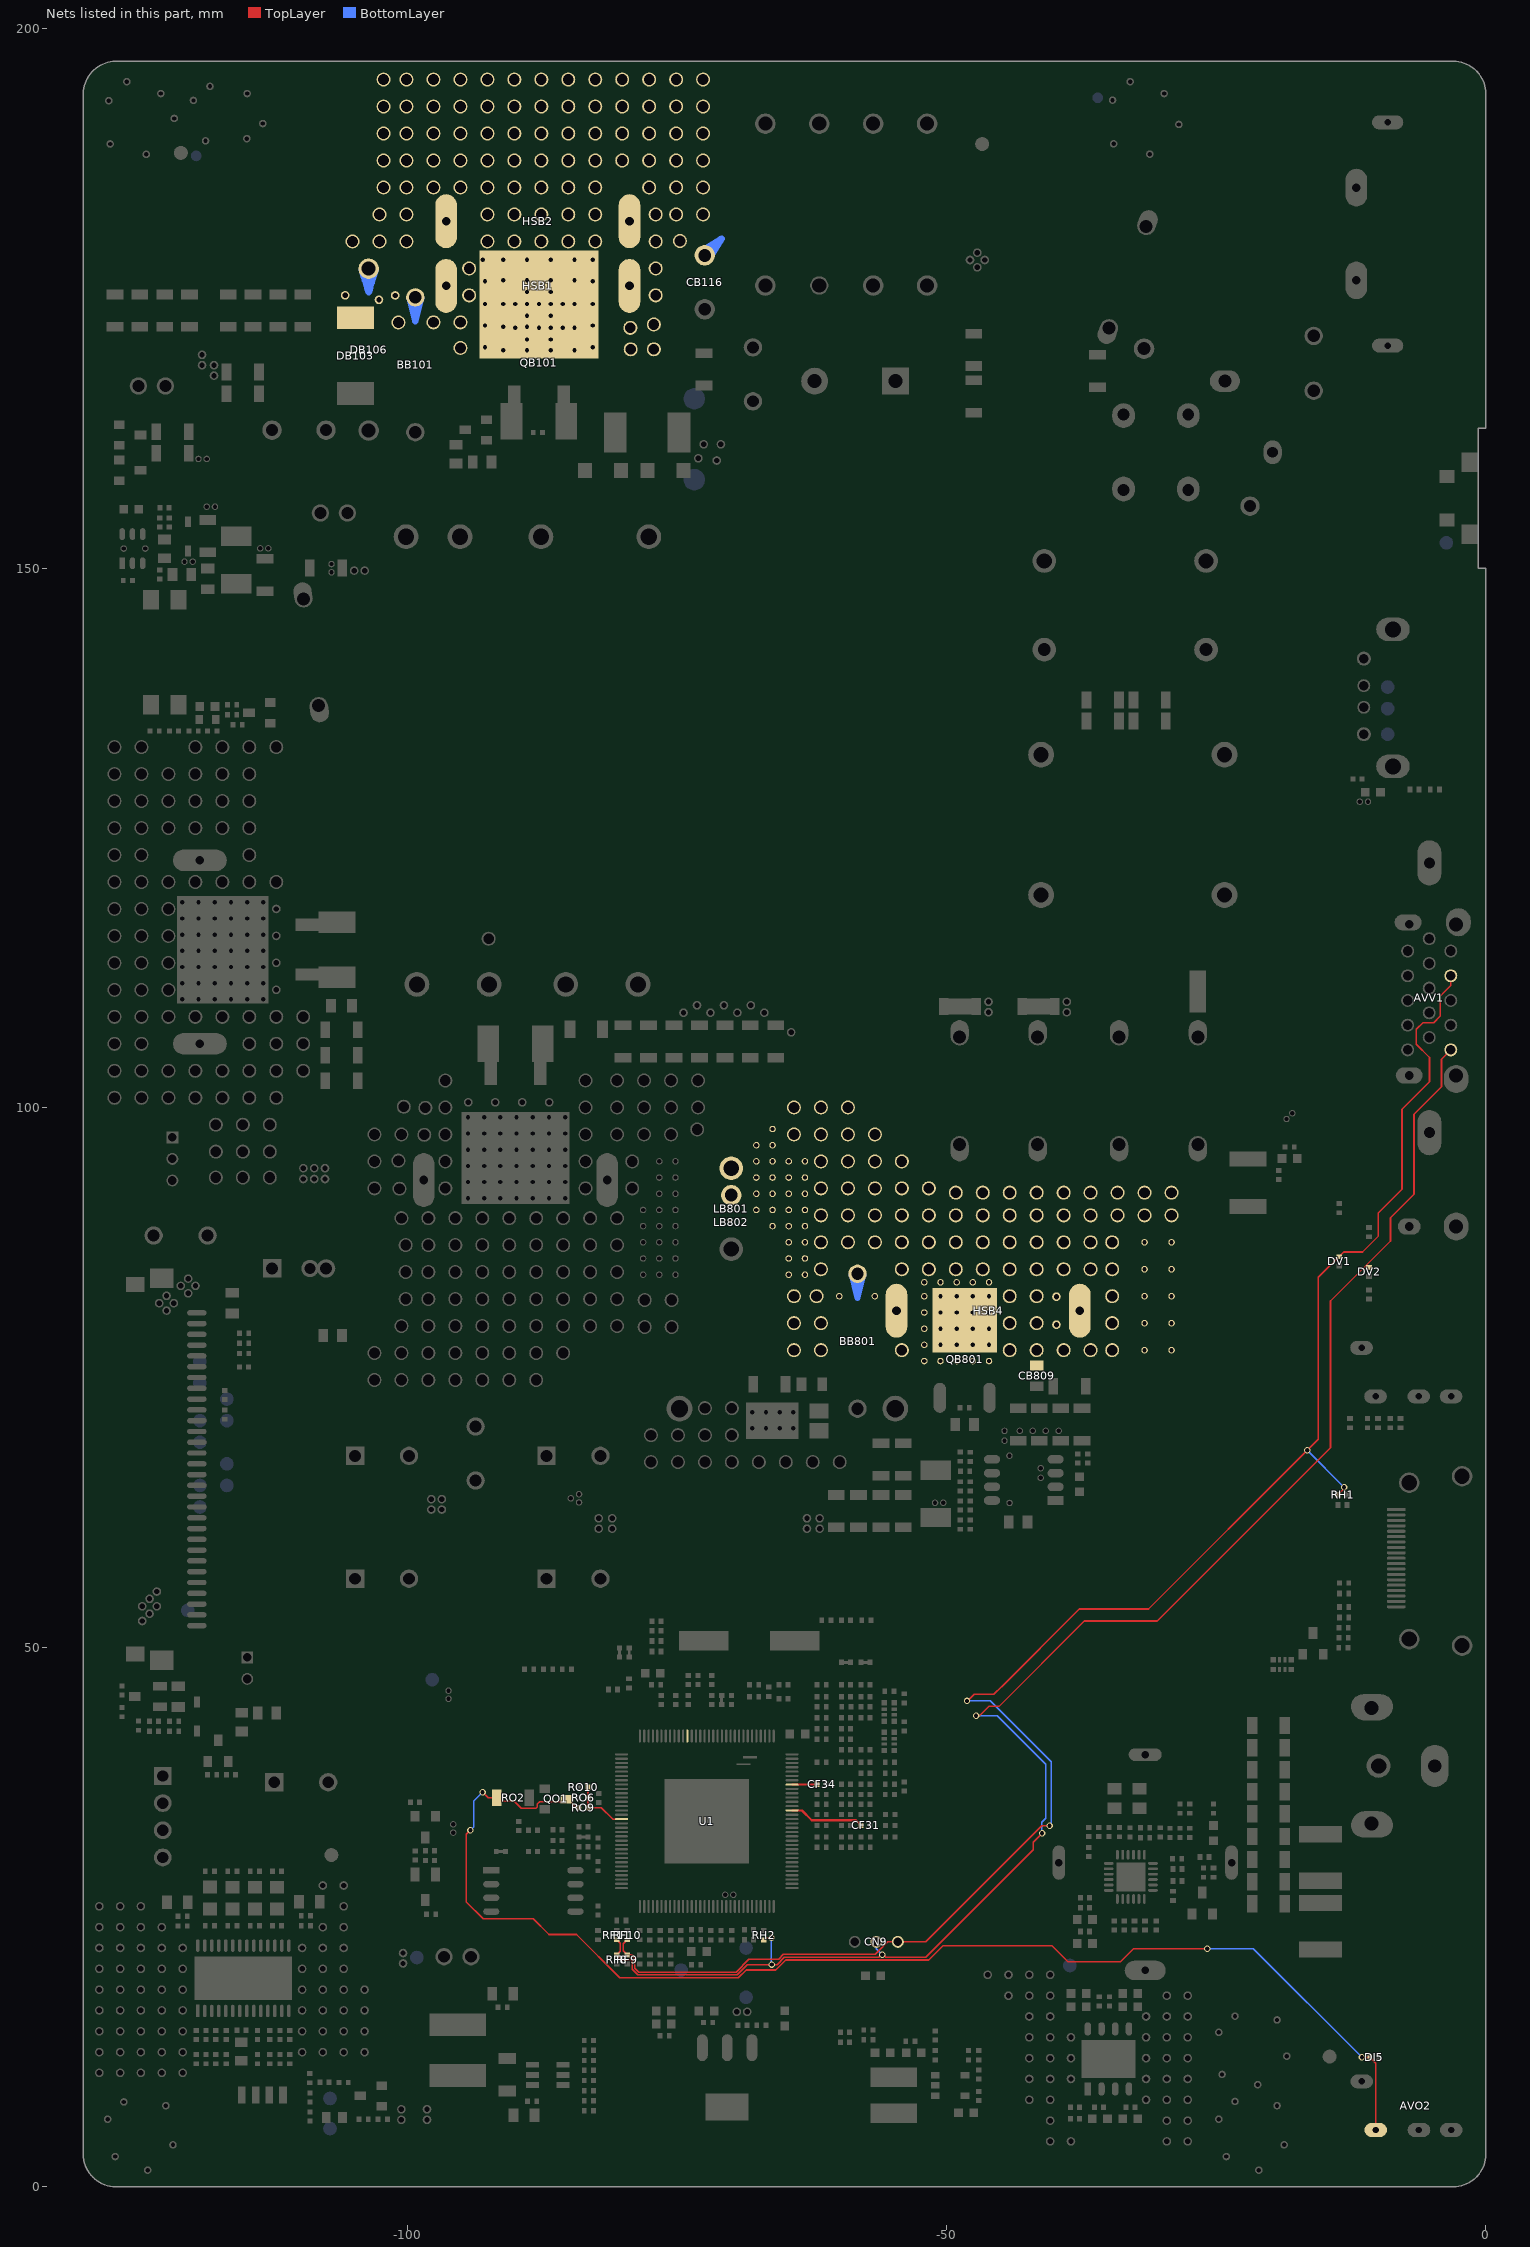
[diagram p0: the nets of this part, all layers, seen from the top]
# Altium PCB MISC84438.PcbDoc (part 8 of 15)
Units mm, origin at the board's own origin, x right, y up, seen from the top; angles counter-clockwise.
Board outline 130 x 197 mm, 2 copper layers (TopLayer, BottomLayer), stack 1.571 mm thick; 574 components, 314 nets, 2636 pads, 811 vias.

## Via types
v1: diameter 0.6, hole 0.4, TopLayer to BottomLayer, tented both sides, 780 vias
v2: diameter 0.7, hole 0.5, TopLayer to BottomLayer, tented both sides, 15 vias
v3: diameter 0.8, hole 0.6, TopLayer to BottomLayer, tented both sides, 12 vias
v4: diameter 0.8, hole 0.5, TopLayer to BottomLayer, tented both sides, 4 vias

## Nets (pads, with @x,y where several pads share a name; then routed paths per layer and width w, separated by ;. In a path a pad name is that pad's centre, name@x,y a point inside that pad or via, vN(x,y) a via of type N, cw(c..) or ccw(c..) an arc to the next point about the centre after c; other vN are vias at no path point) (continued)
D_QB101: BB101.1 CB116.2 DB103.A DB106.A HSB1.1@-79.374,176.188 HSB1.2 HSB2.1@-79.374,182.188 HSB2.2 pad.VIA5@-72.551,182.812 pad.VIA5@-72.551,185.312 pad.VIA5@-72.551,187.812 pad.VIA5@-72.551,190.312 pad.VIA5@-72.551,192.812 pad.VIA5@-72.551,195.312 pad.VIA5@-74.7,180.35 pad.VIA5@-75.051,182.812 pad.VIA5@-75.051,185.312 pad.VIA5@-75.051,187.812 pad.VIA5@-75.051,190.312 pad.VIA5@-75.051,192.812 pad.VIA5@-75.051,195.312 pad.VIA5@-76.951,175.312 pad.VIA5@-76.951,177.812 pad.VIA5@-76.951,180.312 pad.VIA5@-76.951,182.812 pad.VIA5@-77.119,170.312 pad.VIA5@-77.119,172.612 pad.VIA5@-77.551,185.312 pad.VIA5@-77.551,187.812 pad.VIA5@-77.551,190.312 pad.VIA5@-77.551,192.812 pad.VIA5@-77.551,195.312 pad.VIA5@-79.3,172.3 pad.VIA5@-79.264,170.312 pad.VIA5@-80.051,187.812 pad.VIA5@-80.051,190.312 pad.VIA5@-80.051,192.812 pad.VIA5@-80.051,195.312 pad.VIA5@-82.551,180.312 pad.VIA5@-82.551,182.812 pad.VIA5@-82.551,185.312 pad.VIA5@-82.551,187.812 pad.VIA5@-82.551,190.312 pad.VIA5@-82.551,192.812 pad.VIA5@-82.551,195.312 pad.VIA5@-85.051,180.312 pad.VIA5@-85.051,182.812 pad.VIA5@-85.051,185.312 pad.VIA5@-85.051,187.812 pad.VIA5@-85.051,190.312 pad.VIA5@-85.051,192.812 pad.VIA5@-85.051,195.312 pad.VIA5@-87.551,180.312 pad.VIA5@-87.551,182.812 pad.VIA5@-87.551,185.312 pad.VIA5@-87.551,187.812 pad.VIA5@-87.551,190.312 pad.VIA5@-87.551,192.812 pad.VIA5@-87.551,195.312 pad.VIA5@-90.051,180.312 pad.VIA5@-90.051,182.812 pad.VIA5@-90.051,185.312 pad.VIA5@-90.051,187.812 pad.VIA5@-90.051,190.312 pad.VIA5@-90.051,192.812 pad.VIA5@-90.051,195.312 pad.VIA5@-92.551,180.312 pad.VIA5@-92.551,182.812 pad.VIA5@-92.551,185.312 pad.VIA5@-92.551,187.812 pad.VIA5@-92.551,190.312 pad.VIA5@-92.551,192.812 pad.VIA5@-92.551,195.312 pad.VIA5@-94.238,175.312 pad.VIA5@-94.238,177.812 pad.VIA5@-95.051,170.439 pad.VIA5@-95.051,172.812 pad.VIA5@-95.051,185.312 pad.VIA5@-95.051,187.812 pad.VIA5@-95.051,190.312 pad.VIA5@-95.051,192.812 pad.VIA5@-95.051,195.312 pad.VIA5@-97.551,172.812 pad.VIA5@-97.551,185.312 pad.VIA5@-97.551,187.812 pad.VIA5@-97.551,190.312 pad.VIA5@-97.551,192.812 pad.VIA5@-97.551,195.312 pad.VIA5@-100.8,172.8 pad.VIA5@-100.051,180.312 pad.VIA5@-100.051,182.812 pad.VIA5@-100.051,185.312 pad.VIA5@-100.051,187.812 pad.VIA5@-100.051,190.312 pad.VIA5@-100.051,192.812 pad.VIA5@-100.051,195.312 pad.VIA5@-101.1,175.3 pad.VIA5@-102.6,174.9 pad.VIA5@-102.17,185.312 pad.VIA5@-102.17,187.812 pad.VIA5@-102.17,190.312 pad.VIA5@-102.17,192.812 pad.VIA5@-102.17,195.312 pad.VIA5@-102.551,180.312 pad.VIA5@-102.551,182.812 pad.VIA5@-105.051,180.312 pad.VIA5@-105.737,175.312 QB101.2
  other v1: -91.071,170.213 -88.871,170.214 -86.671,170.214 -84.471,170.213 -92.771,170.513 -82.771,170.513 -88.871,171.213 -86.671,171.213 -89.971,172.313 -87.771,172.313 -86.671,172.313 -85.571,172.313 -84.471,172.313 -91.071,172.413 -88.871,172.413 -92.771,172.513 -82.771,172.513 -88.871,173.413 -86.671,173.413 -92.771,174.513 -91.071,174.513 -89.971,174.513 -88.871,174.513 -87.771,174.513 -86.671,174.513 -85.571,174.513 -84.471,174.513 -82.771,174.513 -88.871,175.613 -86.671,175.613 -92.771,176.613 -82.771,176.613 -91.071,176.713 -88.871,176.713 -86.671,176.713 -84.471,176.713 -92.971,178.613 -91.071,178.613 -88.871,178.613 -86.671,178.613 -84.471,178.613 -82.771,178.613
D_QB801: BB801.1 CB809.2 HSB4.1@-54.626,81.193 HSB4.2 LB801.2 LB802.2 pad.VIA5@-29.132,77.536 pad.VIA5@-29.132,80.036 pad.VIA5@-29.132,82.536 pad.VIA5@-29.132,85.036 pad.VIA5@-29.132,87.536 pad.VIA5@-29.132,90.036 pad.VIA5@-29.132,92.136 pad.VIA5@-31.632,77.536 pad.VIA5@-31.632,80.036 pad.VIA5@-31.632,82.536 pad.VIA5@-31.632,85.036 pad.VIA5@-31.632,87.536 pad.VIA5@-31.632,90.036 pad.VIA5@-31.632,92.136 pad.VIA5@-34.132,90.036 pad.VIA5@-34.132,92.136 pad.VIA5@-34.632,77.536 pad.VIA5@-34.632,80.036 pad.VIA5@-34.632,82.536 pad.VIA5@-34.632,85.036 pad.VIA5@-34.632,87.536 pad.VIA5@-36.632,77.536 pad.VIA5@-36.632,85.036 pad.VIA5@-36.632,87.536 pad.VIA5@-36.632,90.036 pad.VIA5@-36.632,92.136 pad.VIA5@-39.8,79.9 pad.VIA5@-39.8,82.5 pad.VIA5@-39.132,77.536 pad.VIA5@-39.132,85.036 pad.VIA5@-39.132,87.536 pad.VIA5@-39.132,90.036 pad.VIA5@-39.132,92.136 pad.VIA5@-41.632,77.536 pad.VIA5@-41.632,80.036 pad.VIA5@-41.632,82.536 pad.VIA5@-41.632,85.036 pad.VIA5@-41.632,87.536 pad.VIA5@-41.632,90.036 pad.VIA5@-41.632,92.136 pad.VIA5@-44.132,77.536 pad.VIA5@-44.132,80.036 pad.VIA5@-44.132,82.536 pad.VIA5@-44.132,85.036 pad.VIA5@-44.132,87.536 pad.VIA5@-44.132,90.036 pad.VIA5@-44.132,92.136 pad.VIA5@-46.05,76.525 pad.VIA5@-46.05,78.025 pad.VIA5@-46.05,79.525 pad.VIA5@-46.05,81.025 pad.VIA5@-46.05,82.525 pad.VIA5@-46.05,83.825 pad.VIA5@-46.632,85.036 pad.VIA5@-46.632,87.536 pad.VIA5@-46.632,90.036 pad.VIA5@-46.632,92.136 pad.VIA5@-47.55,76.525 pad.VIA5@-47.55,78.025 pad.VIA5@-47.55,79.525 pad.VIA5@-47.55,81.025 pad.VIA5@-47.55,82.525 pad.VIA5@-47.55,83.825 pad.VIA5@-49.05,76.525 pad.VIA5@-49.05,78.025 pad.VIA5@-49.05,79.525 pad.VIA5@-49.05,81.025 pad.VIA5@-49.05,82.525 pad.VIA5@-49.05,83.825 pad.VIA5@-49.132,85.036 pad.VIA5@-49.132,87.536 pad.VIA5@-49.132,90.036 pad.VIA5@-49.132,92.136 pad.VIA5@-50.55,76.525 pad.VIA5@-50.55,78.025 pad.VIA5@-50.55,79.525 pad.VIA5@-50.55,81.025 pad.VIA5@-50.55,82.525 pad.VIA5@-50.55,83.825 pad.VIA5@-51.632,85.036 pad.VIA5@-51.632,87.536 pad.VIA5@-51.632,90.036 pad.VIA5@-51.632,92.536 pad.VIA5@-52.05,76.525 pad.VIA5@-52.05,78.025 pad.VIA5@-52.05,79.525 pad.VIA5@-52.05,81.025 pad.VIA5@-52.05,82.525 pad.VIA5@-52.05,83.825 pad.VIA5@-54.131,77.536 pad.VIA5@-54.131,85.036 pad.VIA5@-54.131,87.536 pad.VIA5@-54.131,90.036 pad.VIA5@-54.131,92.536 pad.VIA5@-54.131,95.036 pad.VIA5@-56.631,82.536 pad.VIA5@-56.631,87.536 pad.VIA5@-56.631,90.036 pad.VIA5@-56.631,92.536 pad.VIA5@-56.631,95.036 pad.VIA5@-56.631,97.536 pad.VIA5@-59.131,87.536 pad.VIA5@-59.131,90.036 pad.VIA5@-59.131,92.536 pad.VIA5@-59.131,95.036 pad.VIA5@-59.131,97.536 pad.VIA5@-59.131,100.036 pad.VIA5@-59.931,82.536 pad.VIA5@-61.632,77.536 pad.VIA5@-61.632,80.036 pad.VIA5@-61.632,85.036 pad.VIA5@-61.632,87.536 pad.VIA5@-61.632,90.036 pad.VIA5@-61.632,92.536 pad.VIA5@-61.632,95.036 pad.VIA5@-61.632,97.536 pad.VIA5@-61.632,100.036 pad.VIA5@-62.032,82.536 pad.VIA5@-63.115,84.535 pad.VIA5@-63.115,86.035 pad.VIA5@-63.115,87.535 pad.VIA5@-63.115,89.035 pad.VIA5@-63.115,90.535 pad.VIA5@-63.115,92.035 pad.VIA5@-63.115,93.535 pad.VIA5@-63.115,95.035 pad.VIA5@-64.132,77.536 pad.VIA5@-64.132,80.036 pad.VIA5@-64.132,82.536 pad.VIA5@-64.132,97.536 pad.VIA5@-64.132,100.036 pad.VIA5@-64.615,84.535 pad.VIA5@-64.615,86.035 pad.VIA5@-64.615,87.535 pad.VIA5@-64.615,89.035 pad.VIA5@-64.615,90.535 pad.VIA5@-64.615,92.035 pad.VIA5@-64.615,93.535 pad.VIA5@-64.615,95.035 pad.VIA5@-66.115,89.035 pad.VIA5@-66.115,90.535 pad.VIA5@-66.115,92.035 pad.VIA5@-66.115,93.535 pad.VIA5@-66.115,95.035 pad.VIA5@-66.115,96.535 pad.VIA5@-66.115,98.035 pad.VIA5@-67.615,90.535 pad.VIA5@-67.615,92.035 pad.VIA5@-67.615,93.535 pad.VIA5@-67.615,95.035 pad.VIA5@-67.615,96.535 QB801.D
DDC_SCL/UART_RX: AVV1.15 CN9.2 DV2.K RF8.1 RF11.1 RH2.2 | length 152.8
  TopLayer w0.127: RF11.1@-80.543,22.889 -80.213,22.559 -80.213,21.809 RF8.1@-80.543,21.479 -80.109,21.044 -79.249,21.044 -79.13,20.925 -79.13,20.141 -78.618,19.629 -69.399,19.629 -68.442,20.587 v1(-66.205,20.587) -65.7,20.587 -65.017,21.27 -56.261,21.27 v1@-56.017,21.514 ; RH2.2@-66.916,22.877 -66.717,23.076 v1(-66.214,23.076) ; CN9.2@-56.5,22.403 CN9.2@-56.5,22.687 ; v1@-55.899,21.548 -55.621,21.27 -51.936,21.27 -41.961,31.245 -41.961,31.939 v1(-41.136,32.764)
  TopLayer w0.152: v1(-47.255,43.643) -46.939,43.643 -46.068,44.514 -45.13,44.514 -37.218,52.426 -30.471,52.426 -14.402,68.495 -14.402,80.848 ; -14.402,80.772 -14.402,82.094 -8.839,87.657 -8.839,89.808 -6.655,91.993 -6.655,99.411 -4.103,101.962 -4.103,104.514 AVV1.15@-3.247,105.37
  BottomLayer w0.127: v1@-66.214,20.587 v1(-66.214,23.076) ; CN9.2@-56.5,22.687 -56.5,22.066 v1(-55.94,21.506) ; v1(-47.255,43.643) -45.307,43.643 -40.801,39.137 -40.801,34.14 -41.181,33.76 -41.181,32.809 v1(-41.136,32.764)
DDC_SDA/UART_TX: AVV1.12 CN9.3 DV1.K RF9.1 RF10.1 RH1.2 | length 162.9
  TopLayer w0.127: RF10.1@-79.578,22.889 -79.959,22.508 -79.959,21.854 -79.584,21.479 RF9.1@-79.578,21.479 -79.186,21.479 -78.876,21.168 -78.876,20.246 -78.513,19.883 -69.504,19.883 -68.302,21.085 -65.561,21.085 -65.123,21.524 -56.616,21.524 -55.453,22.687 CN9.3@-54.5,22.687 -51.906,22.687 -41.141,33.452 v1(-40.437,33.452)
  TopLayer w0.152: v1(-48.093,45.018) -48.059,44.984 -47.412,45.631 -45.601,45.631 -44.89,46.342 ; -44.882,46.342 -37.681,53.543 -31.267,53.543 v1(-16.561,68.25) -15.519,69.291 -15.519,84.303 -13.183,86.639 -11.437,86.639 -9.957,88.119 -9.957,90.271 -7.772,92.456 -7.772,99.874 -5.221,102.425 -5.221,104.662 -6.444,105.885 -6.444,107.286 -5.831,107.899 -4.826,107.899 -4.216,108.509 -4.216,110.363 -3.247,111.332 AVV1.12@-3.247,112.24 ; RH1.2@-13.709,64.135 -13.145,64.699 v1(-13.145,64.837)
  BottomLayer w0.127: v1(-48.093,45.018) -45.928,45.018 -40.293,39.383 -40.293,33.595 v1(-40.437,33.452)
  BottomLayer w0.152: v1(-16.561,68.25) -16.558,68.25 v1(-13.145,64.837)
DVD_ON: U1.53
EXE_IR: RO6.2 RO9.2 RO10.2 U1.80 | length 5.4
  TopLayer w0.152: RO10.2@-83.217,37.007 RO6.2@-83.217,36.065 RO9.2@-83.217,35.125 -81.989,35.125 -80.934,34.071 U1.80@-80.112,34.071
EXT_IRO: AVO2.2 DI5.K QO1.C RO2.1 RO9.1 | length 121.3
  TopLayer w0.152: v1(-94.12,33.033) -94.501,32.652 -94.501,26.391 -92.939,24.828 -88.29,24.828 -86.835,23.373 -84.282,23.373 -80.272,19.362 -69.289,19.362 -68.568,20.084 -65.827,20.084 -64.907,21.003 -51.638,21.003 -50.314,22.327 -40.208,22.327 -38.735,20.853 -33.858,20.853 -32.652,22.06 v1(-25.832,22.06) ; v1(-92.996,36.568) -92.471,36.043 RO2.1@-91.67,36.043 ; RO2.1@-91.67,35.714 -90.057,35.714 -89.408,35.064 -88.049,35.064 -87.927,35.187 -87.927,35.47 -87.71,35.687 -85.48,35.687 QO1.C@-85.242,35.926 -85.164,36.003 -84.287,35.125 RO9.1@-84.067,35.125 ; v1(-11.481,11.989) DI5.K@-10.763,11.989 -10.2,11.426 AVO2.2@-10.2,5.25
  BottomLayer w0.152: v1(-94.12,33.033) -93.82,33.333 -93.82,35.744 v1(-92.996,36.568) ; v1(-25.832,22.06) -21.552,22.06 v1(-11.481,11.989)
GIN0N: CF31.1 U1.19 | length 7
  TopLayer w0.198: U1.19@-64.312,34.871 -63.443,34.871
  TopLayer w0.203: -63.443,34.871 -63.395,34.871 -62.48,33.956 -58.384,33.956 CF31.1@-57.905,33.477
GIN1N: CF34.2 U1.25 | length 2.3
  TopLayer w0.198: U1.25@-64.312,37.271 -62.062,37.271 CF34.2@-61.995,37.338